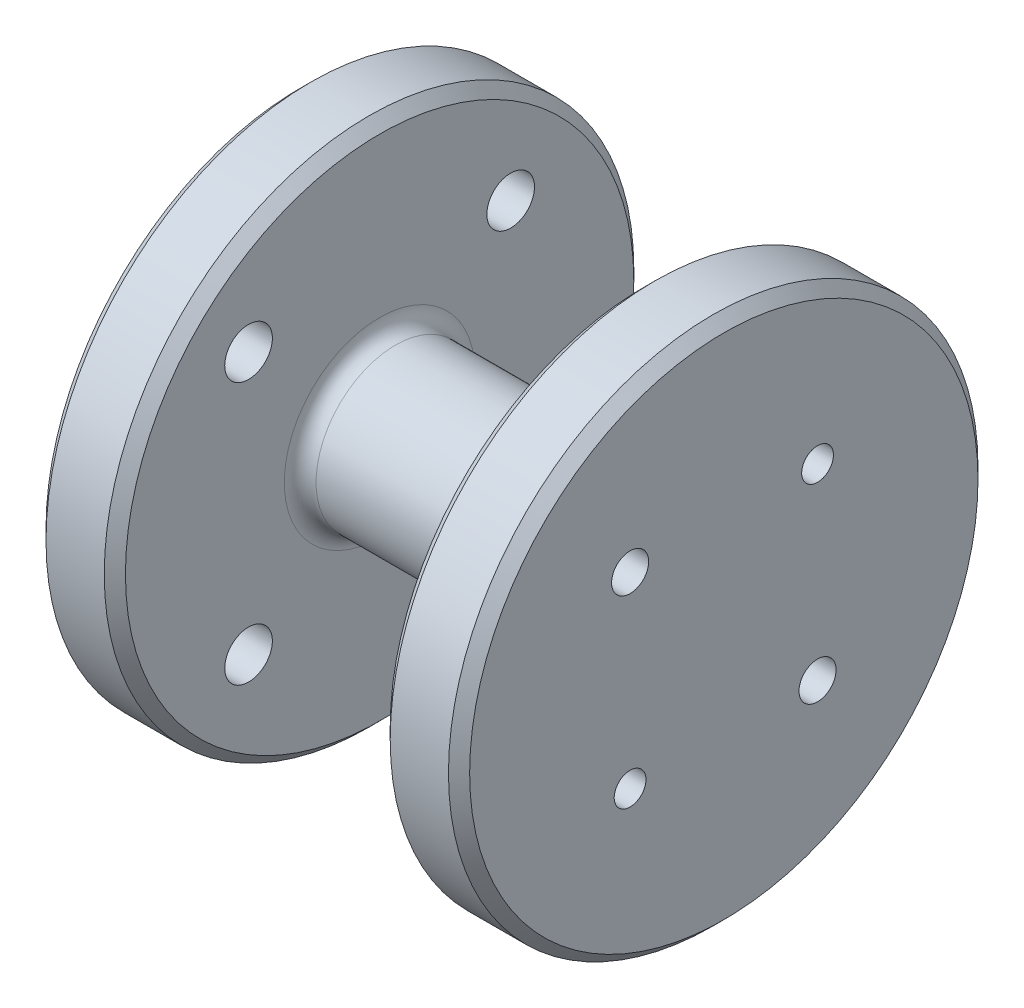
SolidWorks part; units mm, degrees
ref_plane "前视基准面" through (0, 0, 0) normal (0, 0, 1) x (1, 0, 0)
ref_plane "上视基准面" through (0, 0, 0) normal (0, 1, 0) x (1, 0, 0)
ref_plane "右视基准面" through (0, 0, 0) normal (1, 0, 0) x (0, 0, -1)
sketch "草图1" plane through (0, 0, 0) normal (1, 0, 0) x (0, 0, -1)
  circle A0 centre (0, 0) radius 50
  dimension "D1" = 100
extrude "凸台-拉伸1" add sketch "草图1" along normal blind 15
sketch "草图2" plane through (15, 0, 0) normal (1, 0, 0) x (0, 0, -1)
  circle A0 centre (0, 0) radius 15
  dimension "D1" = 30
extrude "凸台-拉伸2" add sketch "草图2" along normal blind 50
sketch "草图3" plane through (65, 0, 0) normal (1, 0, 0) x (0, 0, -1)
  circle A0 centre (0, 0) radius 50
  dimension "D1" = 100
extrude "凸台-拉伸3" add sketch "草图3" along normal blind 15
hole_wizard "Ø7.0 (7) 直径孔1" positions "草图4" profile "草图5" hole size "Ø7.0" standard "GB"
sketch "草图4" plane through (80, 0, 0) normal (1, 0, 0) x (0, 0, -1)
  line L0 (-17.6989, 17.6989) -> (17.6989, -17.6989) construction
  line L2 (0, 0) -> (0, 21.9323) construction
  circle A0 centre (0, 0) radius 25.03 construction
  point P0 (-17.6989, 17.6989)
  point P2 (17.6989, -17.6989)
  dimension "D1" = 50.06
  dimension "D2" = 45
sketch "草图5" plane through (80, 17.6989, 17.6989) normal (0, 1, 0) x (0, 0, -1)
  line L0 (0, 0) -> (0, 21.853)
  line L1 (0, 21.853) -> (3.5, 19.75)
  line L2 (3.5, 19.75) -> (3.5, 0)
  line L5 (3.5, 0) -> (0, 0)
  line L10 (0, 21.853) -> (-3.5, 19.75) construction
  line L11 (0, -6.35) -> (0, 107.95) construction
  dimension "孔直径" = 7
  dimension "孔深度" = 19.75
  dimension "导头角度" = 118
hole_wizard "大小mm 暗销孔1" positions "草图6" profile "草图7" hole size "Ø6.0" standard "GB"
sketch "草图6" plane through (80, 0, 0) normal (1, 0, 0) x (0, 0, -1)
  line L0 (-17.6989, -17.6989) -> (17.6989, 17.6989) construction
  line L2 (0, 0) -> (0, 27.425) construction
  circle A0 centre (0, 0) radius 25.03 construction
  point P0 (-17.6989, -17.6989)
  point P2 (17.6989, 17.6989)
  dimension "D1" = 45
sketch "草图7" plane through (80, -17.6989, 17.6989) normal (0, 1, 0) x (0, 0, -1)
  line L0 (0, 0) -> (0, 21.5526)
  line L1 (0, 21.5526) -> (3, 19.75)
  line L2 (3, 19.75) -> (3, 0)
  line L5 (3, 0) -> (0, 0)
  line L10 (0, 21.5526) -> (-3, 19.75) construction
  line L11 (0, -6.35) -> (0, 107.95) construction
  dimension "孔直径" = 6
  dimension "孔深度" = 19.75
  dimension "导头角度" = 118
hole_wizard "Ø9.0 (9) 直径孔1" positions "草图8" profile "草图9" hole size "Ø9.0" standard "GB"
sketch "草图8" plane through (0, 0, 0) normal (-1, 0, 0) x (0, 0, 1)
  line L0 (-24.7487, 24.7487) -> (0, 0) construction
  line L1 (0, 0) -> (0, 36.2111) construction
  point P0 (-24.7487, 24.7487)
  dimension "D1" = 45
  dimension "D2" = 35
sketch "草图9" plane through (0, 24.7487, -24.7487) normal (0, 1, 0) x (0, 0, 1)
  line L0 (0, 0) -> (0, 22.4539)
  line L1 (0, 22.4539) -> (4.5, 19.75)
  line L2 (4.5, 19.75) -> (4.5, 0)
  line L5 (4.5, 0) -> (0, 0)
  line L10 (0, 22.4539) -> (-4.5, 19.75) construction
  line L11 (0, -6.35) -> (0, 107.95) construction
  dimension "孔直径" = 9
  dimension "孔深度" = 19.75
  dimension "导头角度" = 118
pattern_circular "阵列(圆周)1" count 4 over 360 about axis through (0, 0, 0) along (1, 0, 0) of "Ø9.0 (9) 直径孔1"
fillet "圆角1" radius 3 2 edges at (15, 0, -15) (65, 0, -15)
chamfer "倒角1" distance 2 angle 45 4 edges at (0, 0, -50) (15, 0, -50) (65, 0, -50) (80, 0, -50)
